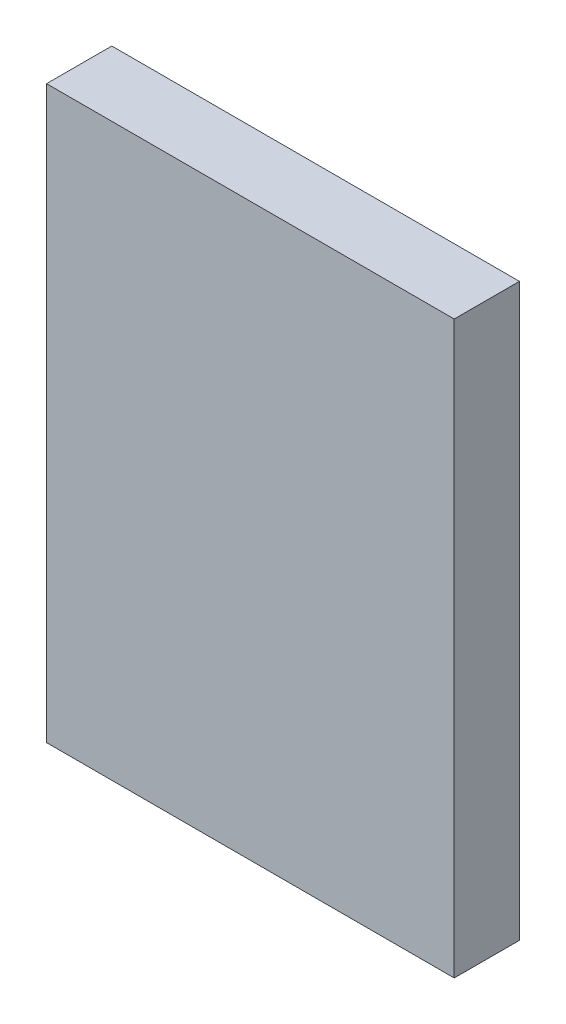
from build123d import *

# Parameters (mm, degrees)
SKETCH_1_W      = 50
SKETCH_1_H      = 70
EXTRUDE_1_DEPTH = 4


with BuildPart() as part:
    # 草图1 → 凸台-拉伸1 (new, symmetric)
    with BuildSketch(Plane.XY):
        Rectangle(SKETCH_1_W, SKETCH_1_H)
    extrude(amount=EXTRUDE_1_DEPTH, both=True)


solid = part.part
